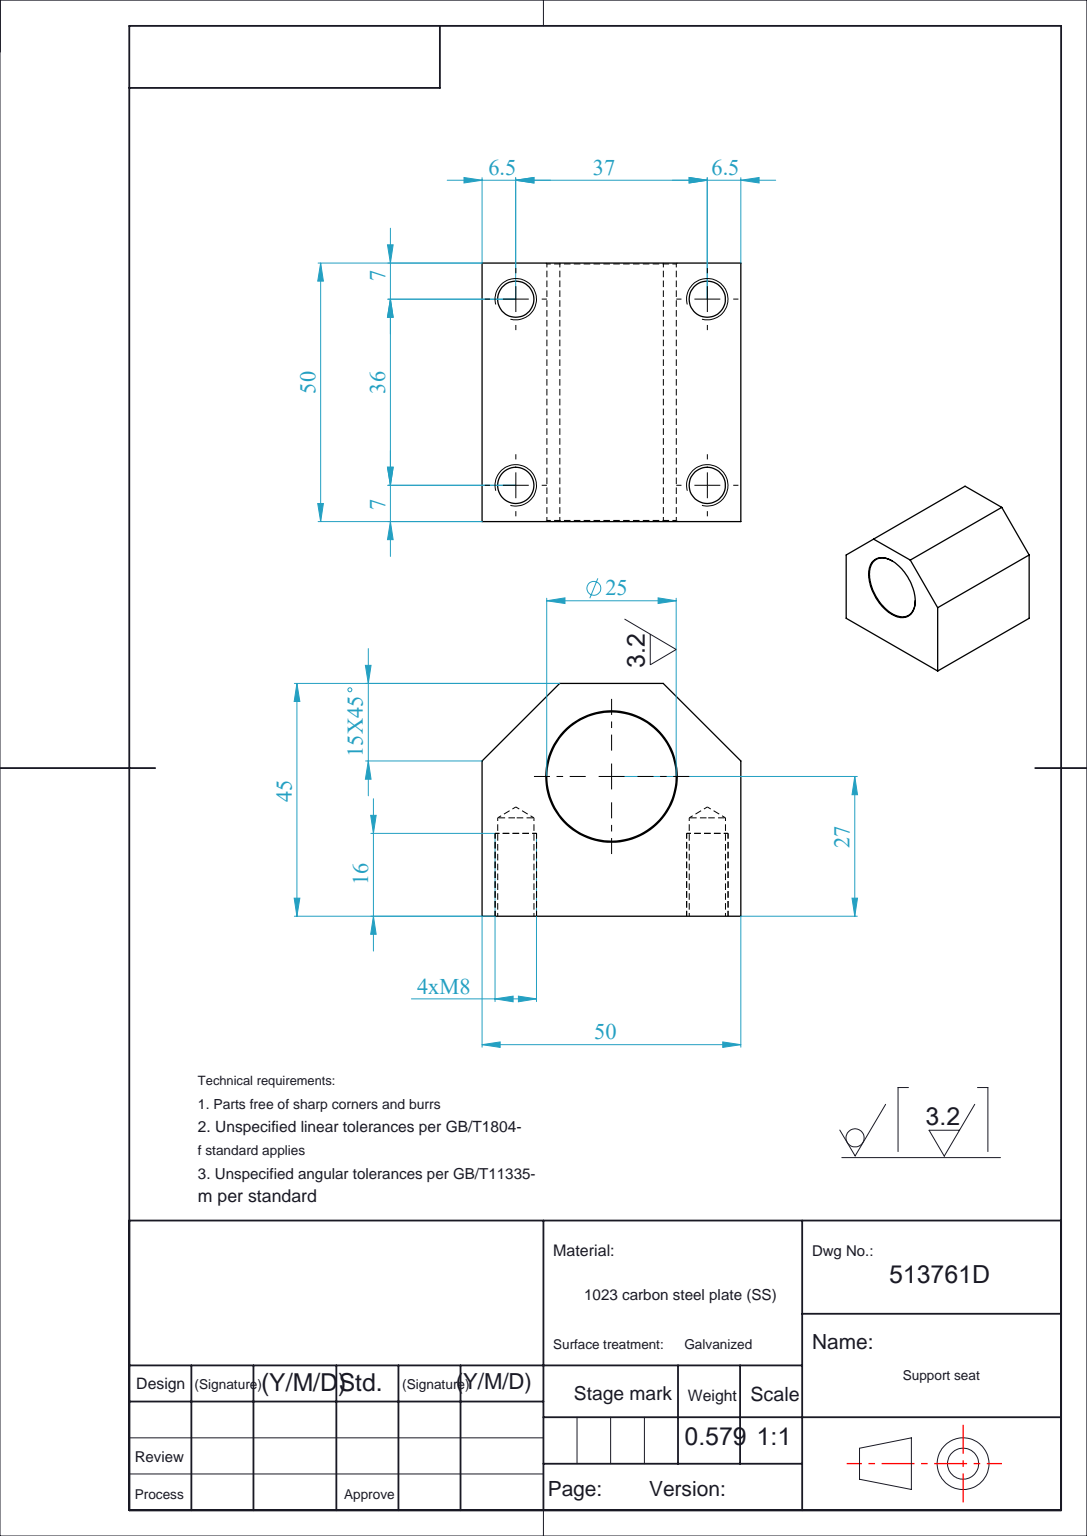
SolidWorks part; units mm, degrees
material "1023 碳钢板 (SS)"
ref_plane "Front Plane" through (0, 0, 0) normal (0, 0, 1) x (1, 0, 0)
ref_plane "Top Plane" through (0, 0, 0) normal (0, 1, 0) x (1, 0, 0)
ref_plane "Right Plane" through (0, 0, 0) normal (1, 0, 0) x (0, 0, -1)
sketch "Sketch1" plane through (0, 0, 0) normal (0, 0, 1) x (1, 0, 0)
  line L1 (-25, 25) -> (25, 25)
  line L2 (-25, 25) -> (-25, -25)
  line L3 (-25, -25) -> (25, -25)
  line L4 (25, 25) -> (25, -25)
  line L5 (-25, 25) -> (25, -25) construction
  line L6 (-25, -25) -> (25, 25) construction
  point P0 (0, 0)
  dimension "D1" = 50
  dimension "D2" = 50
extrude "Boss-Extrude1" add sketch "Sketch1" along normal blind 45
sketch "Sketch3" plane through (25, 0, 0) normal (1, 0, 0) x (0, 0, -1)
  line L0 (0, -25) -> (0, 25) construction
  circle A0 centre (-27, 0) radius 12.5
  dimension "D1" = 25
  dimension "D2" = 27
extrude "Cut-Extrude1" cut sketch "Sketch3" against normal blind 56
chamfer "Chamfer1" distance 15 angle 45 2 edges at (0, 25, 45) (0, -25, 45)
sketch "Sketch4" plane through (0, 0, 0) normal (0, 0, -1) x (-1, 0, 0)
  line L0 (-25, -25) -> (-25, 25) construction
  line L1 (-25, 25) -> (25, 25) construction
  circle A0 centre (-18, 18.5) radius 4
  circle A1 centre (18, 18.5) radius 4
  circle A2 centre (-18, -18.5) radius 4
  circle A3 centre (18, -18.5) radius 4
  dimension "D5" = 8
  dimension "D1" = 7
  dimension "D2" = 6.5
  dimension "D3" = 36
  dimension "D4" = 37
hole_wizard "M8x1.0 Tapped Hole1" positions "Sketch9" profile "Sketch10" tap size "M8x1.0" standard "GB"
sketch "Sketch9" plane through (0, 0, 0) normal (0, 0, -1) x (-1, 0, 0)
  point P0 (-18, 18.5)
  point P3 (18, 18.5)
  point P6 (18, -18.5)
  point P9 (-18, -18.5)
sketch "Sketch10" plane through (18, 18.5, 0) normal (1, 0, 0) x (0, 1, 0)
  line L0 (0, 0) -> (0, 21.103)
  line L1 (0, 21.103) -> (3.5, 19)
  line L2 (3.5, 19) -> (3.5, 0)
  line L5 (3.5, 0) -> (0, 0)
  line L10 (0, 21.103) -> (-3.5, 19) construction
  line L11 (0, -6.35) -> (0, 107.95) construction
  dimension "螺纹孔钻头直径" = 7
  dimension "螺纹孔钻头深度" = 19
  dimension "导头角度" = 118
cosmetic thread "Cosmetic Thread5"
cosmetic thread "Cosmetic Thread6"
cosmetic thread "Cosmetic Thread7"
cosmetic thread "Cosmetic Thread8"
chamfer "Chamfer2" distance 0.2 angle 45 1 edges at (25, 12.5, 27)
chamfer "Chamfer3" distance 0.2 angle 45 1 edges at (-25, 12.5, 27)
